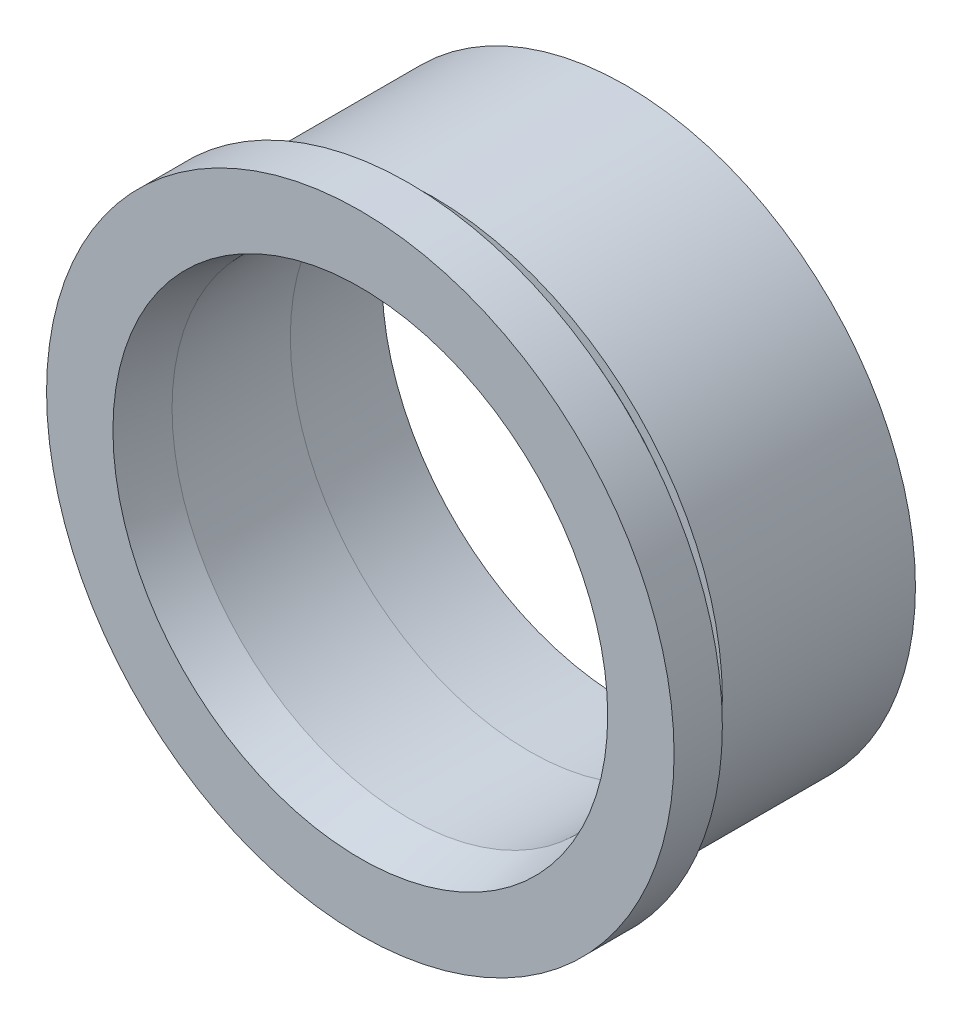
from build123d import *


with BuildPart() as part:
    # Sketch1 → Revolve1 (revolve)
    with BuildSketch(Plane(origin=(0, 234.743963655, 0), x_dir=(1, 0, 0), z_dir=(0, 1, 0))):
        Polygon((586.230642584, 1054.692956355), (579.230642584, 1054.692956355), (579.230642584, 1059.692956355), (581.230642584, 1059.692956355), (581.230642584, 1099.692956355), (571.730642584, 1099.692956355), (570.730642584, 1079.692956355), (570.230642584, 1054.692956355), (572.480642584, 1044.692956355), (586.230642584, 1044.692956355), align=None)
    revolve(axis=Axis((521.230642584, 234.743963655, -1099.692956355), (0, 0, 1)))


solid = part.part
